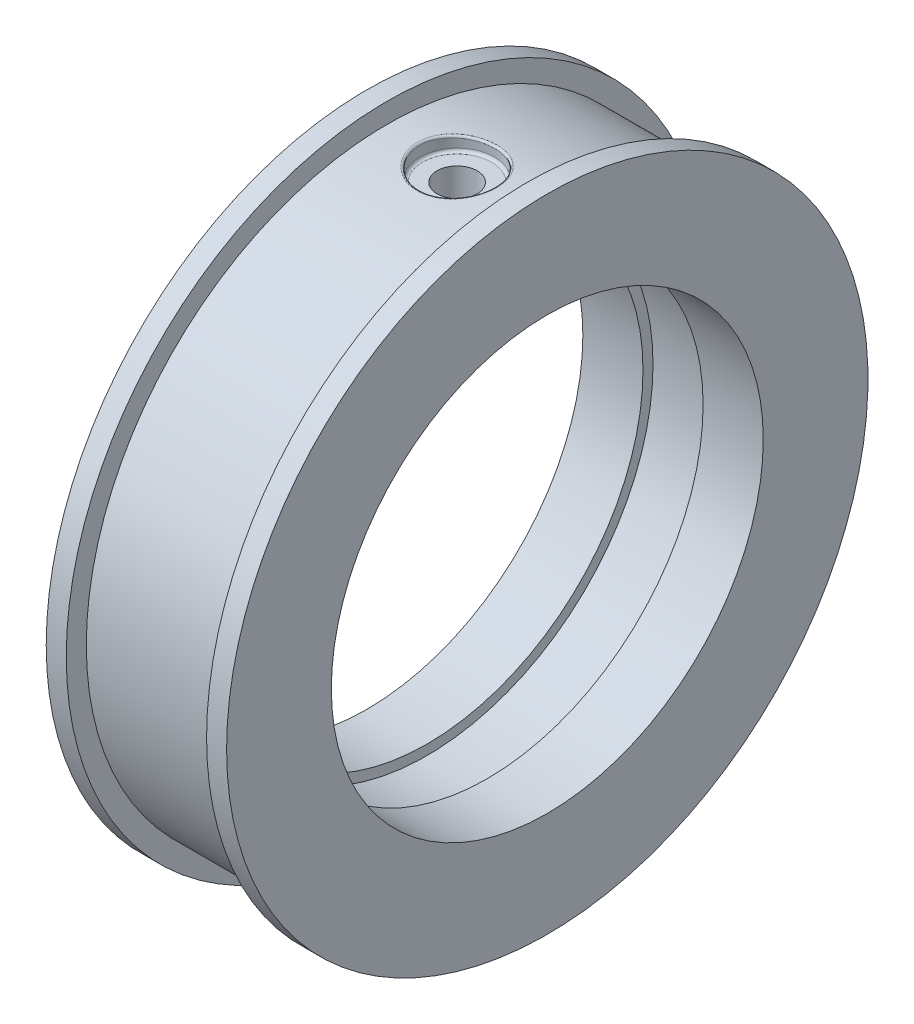
SolidWorks part; units mm, degrees
ref_plane "Front Plane" through (0, 0, 0) normal (0, 0, 1) x (1, 0, 0)
ref_plane "Top Plane" through (0, 0, 0) normal (0, 1, 0) x (1, 0, 0)
ref_plane "Right Plane" through (0, 0, 0) normal (1, 0, 0) x (0, 0, -1)
sketch "Sketch1" plane through (0, 0, 0) normal (0, 0, 1) x (1, 0, 0)
  line L0 (-19.0368, 0) -> (19.2228, 0) construction
  line L1 (-8.3897, 21.55) -> (-8.3897, 32)
  line L2 (-8.3897, 32) -> (-6.3897, 32)
  line L3 (-6.3897, 32) -> (-6.3897, 30)
  line L4 (-6.3897, 30) -> (7.6103, 30)
  line L5 (7.6103, 30) -> (7.6103, 32)
  line L6 (7.6103, 32) -> (9.6103, 32)
  line L7 (9.6103, 32) -> (9.6103, 21.55)
  line L8 (9.6103, 21.55) -> (3.6103, 21.55)
  line L9 (3.6103, 21.55) -> (3.6103, 22.55)
  line L10 (3.6103, 22.55) -> (-2.3897, 22.55)
  line L11 (-2.3897, 22.55) -> (-2.3897, 21.55)
  line L12 (-2.3897, 21.55) -> (-8.3897, 21.55)
  dimension "D2" = 18
  dimension "D3" = 14
  dimension "D4" = 2
  dimension "D5" = 21.55
  dimension "D6" = 21.55
  dimension "D7" = 22.55
  dimension "D8" = 6
  dimension "D9" = 6
  dimension "D10" = 30
  dimension "D11" = 32
  dimension "D12" = 32
revolve "Revolve1" add sketch "Sketch1" angle 360 about L0
ref_plane "Plane1" through (0, 30, 0) normal (0, 1, 0) x (1, 0, 0)
sketch "Sketch2" plane through (0, 30, 0) normal (0, 1, 0) x (1, 0, 0)
  line L0 (-6.3897, 0) -> (7.6103, 0)
  line L1 (-6.3897, -32) -> (-6.3897, 32) construction
  line L2 (7.6103, 30) -> (7.6103, -30) construction
hole_wizard "Hole1" positions "Sketch3" profile "Sketch4" legacy
sketch "Sketch3" plane through (0, 30, 0) normal (0, 1, 0) x (1, 0, 0)
  line L0 (-6.3897, 0) -> (7.6103, 0) construction
  point P0 (0.6103, 0)
sketch "Sketch4" plane through (0.6103, 30, 0) normal (1, 0, 0) x (0, 0, 1)
  line L0 (0, 0) -> (0, 1.5)
  line L1 (0, 1.5) -> (3.75, 1.5)
  line L2 (3.75, 1.5) -> (3.75, 0)
  line L3 (3.75, 0) -> (0, 0)
  line L4 (0, 110) -> (0, -10) construction
  dimension "直径" = 7.5
  dimension "深度" = 1.5
hole_wizard "Hole2" positions "Sketch5" profile "Sketch6" legacy
sketch "Sketch5" plane through (0, 28.5, 0) normal (0, 1, 0) x (1, 0, 0)
  point P0 (0.6103, 0)
sketch "Sketch6" plane through (0.6103, 28.5, 0) normal (1, 0, 0) x (0, 0, 1)
  line L0 (0, 0) -> (0, 5.95)
  line L1 (0, 5.95) -> (2, 5.95)
  line L2 (2, 5.95) -> (2, 0)
  line L3 (2, 0) -> (0, 0)
  line L4 (0, 110) -> (0, -10) construction
  dimension "直径" = 4
  dimension "深度" = 5.95
ref_plane "Plane2" through (0, -30, 0) normal (0, -1, 0) x (-1, 0, 0)
sketch "Sketch8" plane through (0, -30, 0) normal (0, -1, 0) x (-1, 0, 0)
  line L0 (6.3897, 0) -> (-7.6103, 0) construction
  line L1 (6.3897, 0) -> (-7.6103, 0)
hole_wizard "Dowel Hole1" positions "Sketch9" profile "Sketch10" hole size "Ø4.0" standard "GB"
sketch "Sketch9" plane through (0, -30, 0) normal (0, -1, 0) x (-1, 0, 0)
  line L0 (6.3897, 0) -> (-7.6103, 0) construction
  point P0 (-0.6103, 0)
sketch "Sketch10" plane through (0.6103, -30, 0) normal (1, 0, 0) x (0, 0, -1)
  line L0 (0, 0) -> (0, 5.2017)
  line L1 (0, 5.2017) -> (2, 4)
  line L2 (2, 4) -> (2, 0)
  line L5 (2, 0) -> (0, 0)
  line L10 (0, 5.2017) -> (-2, 4) construction
  line L11 (0, -6.35) -> (0, 107.95) construction
  dimension "孔直径" = 4
  dimension "孔深度" = 4
  dimension "导头角度" = 118
fillet "Fillet1" radius 0.2 1 edges at (1.44, 29.7763, -3.6571)
fillet "Fillet2" radius 0.3 1 edges at (0.6103, 28.5, 3.75)
